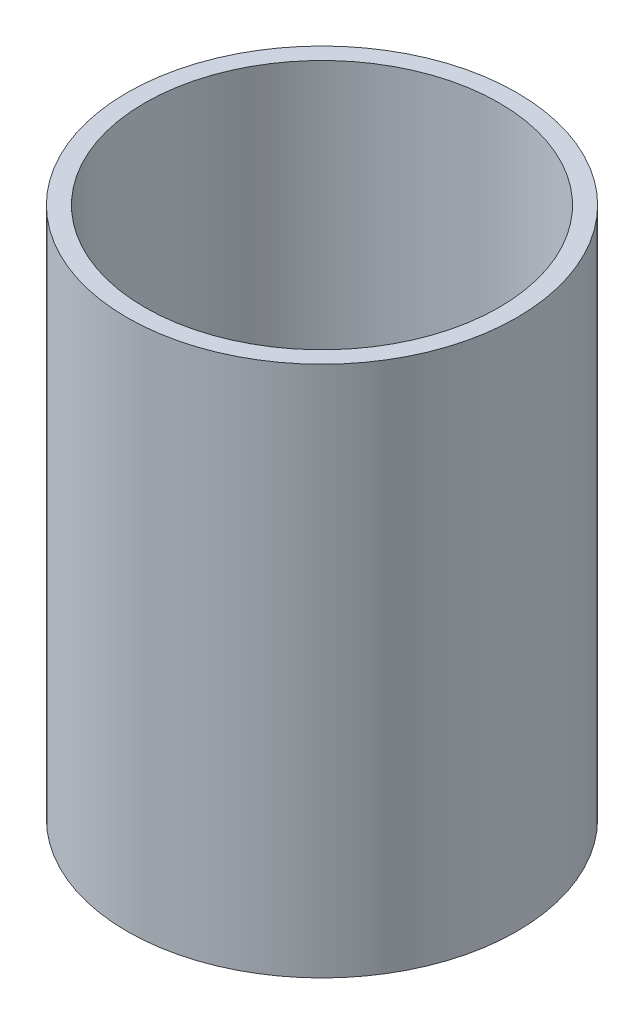
SolidWorks part; units mm, degrees
ref_plane "Front Plane" through (0, 0, 0) normal (0, 0, 1) x (1, 0, 0)
ref_plane "Top Plane" through (0, 0, 0) normal (0, 1, 0) x (1, 0, 0)
ref_plane "Right Plane" through (0, 0, 0) normal (1, 0, 0) x (0, 0, -1)
sketch "Sketch1" plane through (0, 0, 0) normal (0, 1, 0) x (1, 0, 0)
  circle A0 centre (0, 0) radius 110
  dimension "D1" = 220
extrude "Boss-Extrude1" add sketch "Sketch1" along normal blind 300
sketch "Sketch3" plane through (0, 0, 0) normal (0, -1, 0) x (1, 0, 0)
  circle A0 centre (0, 0) radius 100
  dimension "D1" = 200
extrude "Cut-Extrude1" cut sketch "Sketch3" against normal blind 20
sketch "Sketch4" plane through (0, 300, 0) normal (0, 1, 0) x (1, 0, 0)
  circle A0 centre (0, 0) radius 100
  dimension "D1" = 200
extrude "Cut-Extrude2" cut sketch "Sketch4" against normal blind 270
